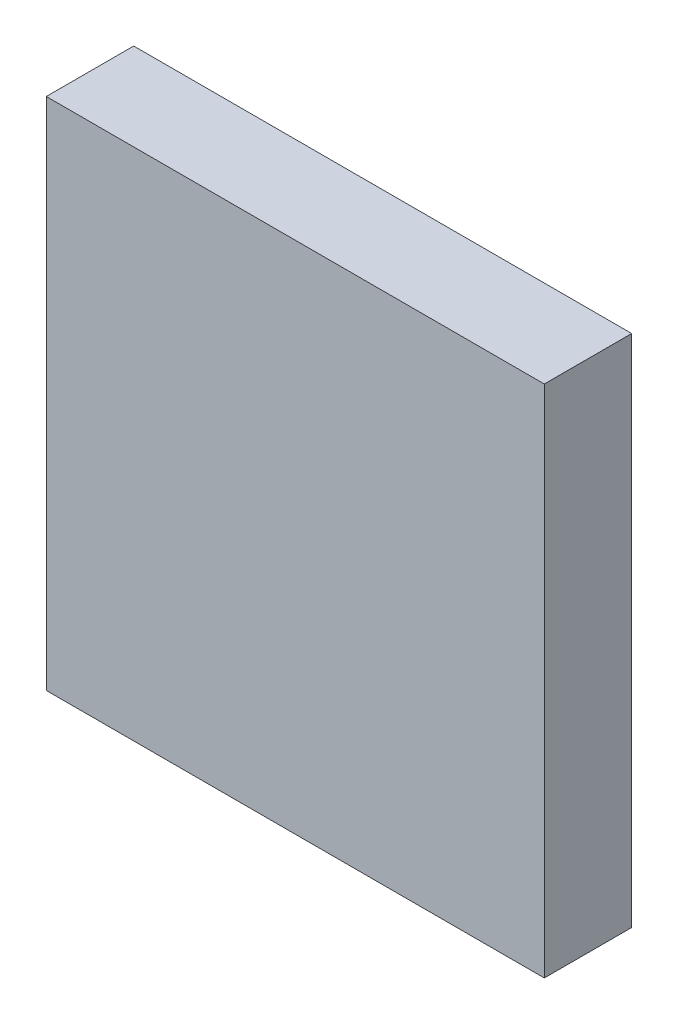
SolidWorks part; units mm, degrees
ref_plane "前视基准面" through (0, 0, 0) normal (0, 0, 1) x (1, 0, 0)
ref_plane "上视基准面" through (0, 0, 0) normal (0, 1, 0) x (1, 0, 0)
ref_plane "右视基准面" through (0, 0, 0) normal (1, 0, 0) x (0, 0, -1)
sketch "草图1" plane through (0, 0, 0) normal (0, 0, 1) x (1, 0, 0)
  line L1 (-28.4844, 29.4249) -> (28.4844, 29.4249)
  line L2 (-28.4844, 29.4249) -> (-28.4844, -29.4249)
  line L3 (-28.4844, -29.4249) -> (28.4844, -29.4249)
  line L4 (28.4844, 29.4249) -> (28.4844, -29.4249)
  line L5 (-28.4844, 29.4249) -> (28.4844, -29.4249) construction
  line L6 (-28.4844, -29.4249) -> (28.4844, 29.4249) construction
  point P0 (0, 0)
extrude "凸台-拉伸1" add sketch "草图1" against normal blind 10
